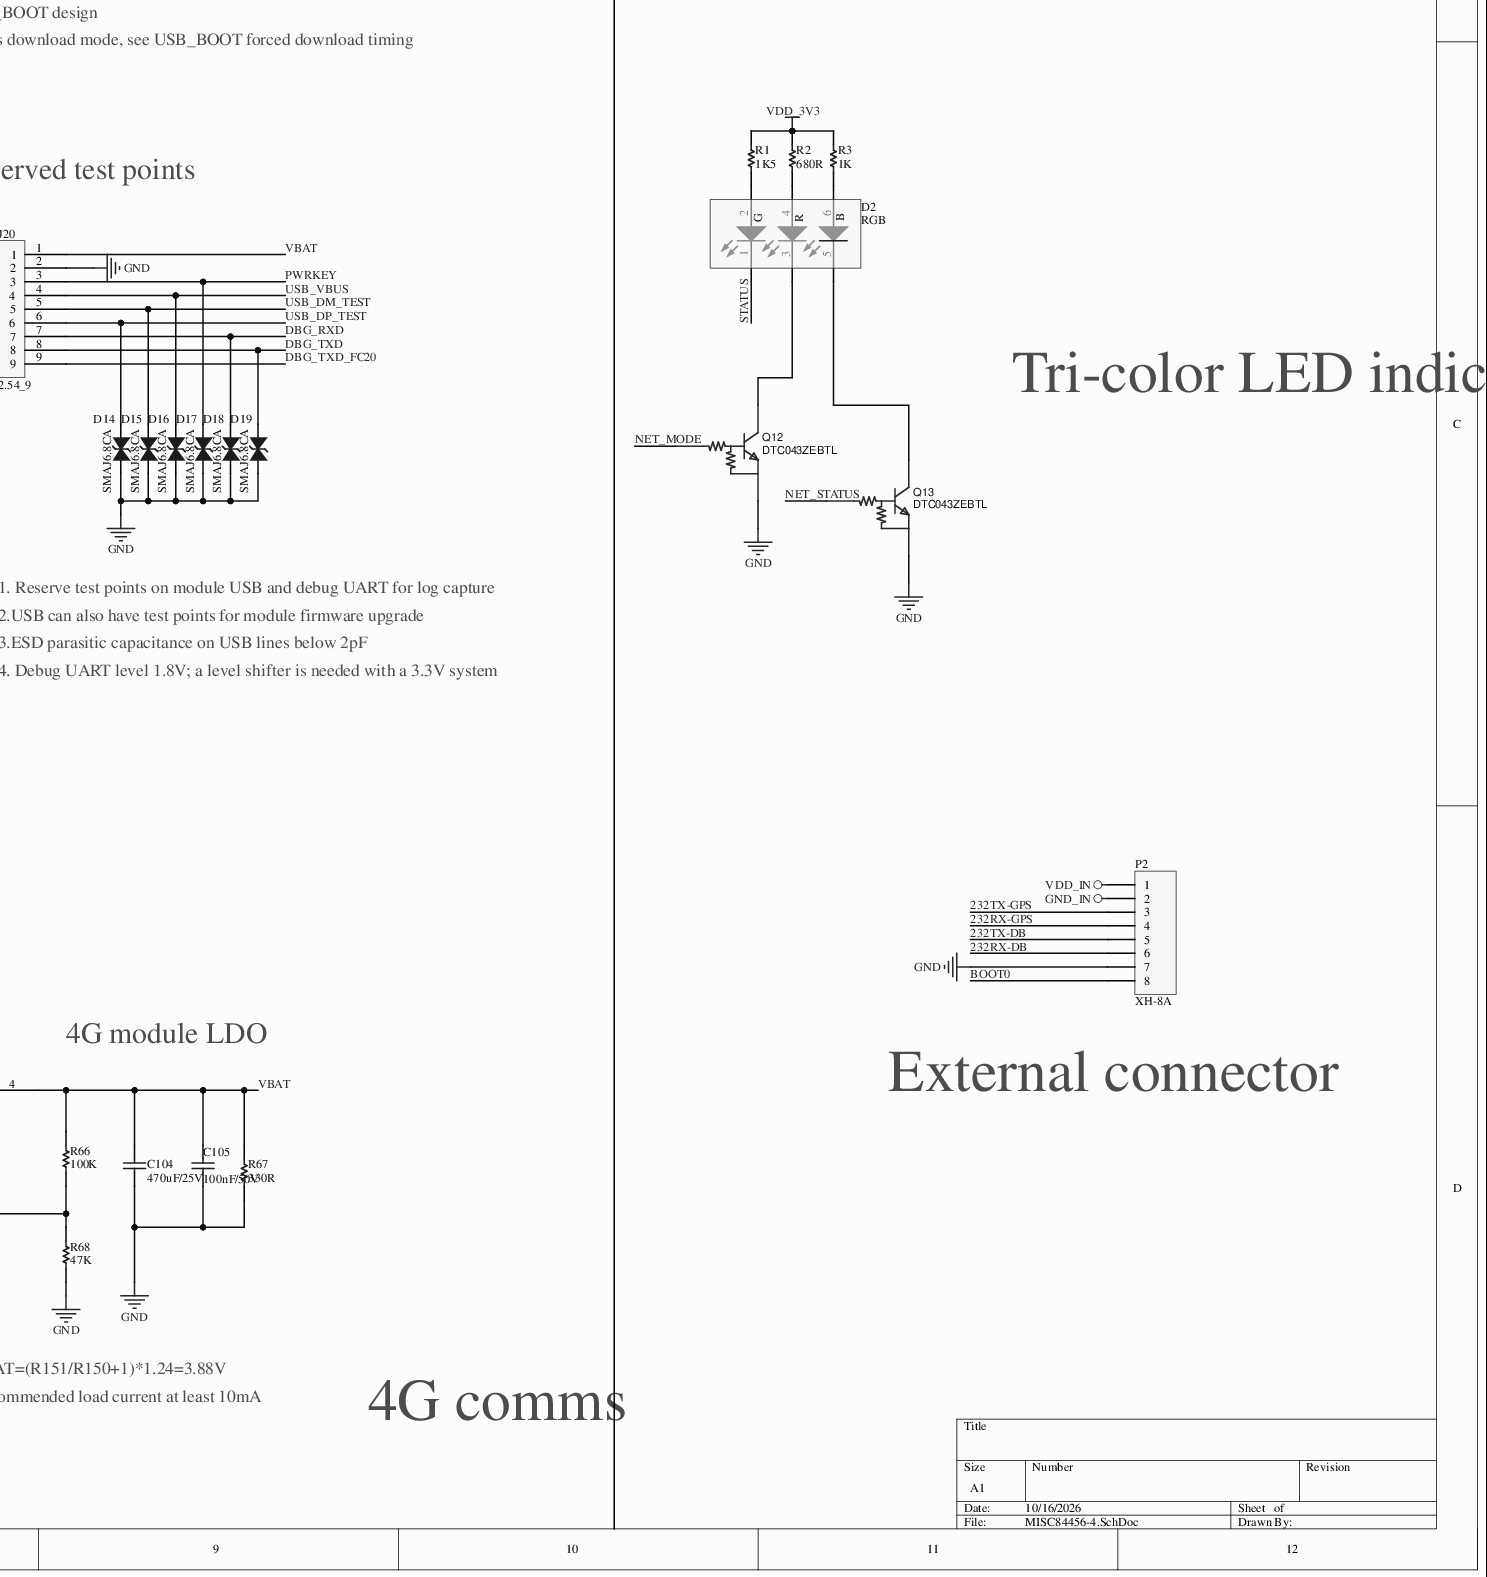
[diagram p0: MISC84456-4.SchDoc, bottom right]
# Altium project MISC84456-3.PrjPcb (part 2 of 2)

## Sheet MISC84456-4.SchDoc
size A1

### Parts
C1  100nF/50V  [C0603]
C2  100nF/50V  [C0603]
C3  100nF/50V  [C0603]  (value not drawn)
C4  470uF/25V  [RB8*11.5]
C5  10uF/25V±10%  [C1206]
C6  100nF/50V  [C0603]
C7  100pF  [C0603]
C8  100pF  [C0603]
C9  100nF/50V  [C0603]
C10  10uF/25V±10%  [C1206]
C11  100nF/50V  [C0603]  (value not drawn)
C20  100pF  [C0603]
C21  100nF/50V  [C0603]
C22  10uF/25V±10%  [C1206]
C23  100nF/50V  [C0603]
C24  100nF/50V  [C0603]
C25  100pF  [C0603]
C26  22uF/10V±20%  [C0805]
C27  100nF/50V  [C0603]
C28  22uF/10V±20%  [C0805]
C29  100uF/10V  [RB5*7]
C30  10uF/25V±10%  [C1206]
C31  100nF/50V  [C0603]
C32  10nF/50V  [C0603]
C33  100nF/50V  [C0603]
C34  33pF/50V  [C0603]
C35  33pF/50V  [C0603]
C36  33pF/50V  [C0603]
C37  33pF/50V  [C0603]
C38  100nF/50V  [C0603]
C39  100pF  [C0603]
C40  22uF/10V±20%  [C0805]
C41  100nF/50V  [C0603]
C42  22uF/10V±20%  [C0805]
C43  22uF/10V±20%  [C0805]
C44  10uF/25V±10%  [C1206]
C45  100nF/50V  [C0603]
C46  100nF/50V  [C0603]
C47  10nF/50V  [C0603]
C48  10nF/50V  [C0603]
C49  33pF/50V  [C0603]
C50  33pF/50V  [C0603]
C51  33pF/50V  [C0603]
C52  33pF/50V  [C0603]
C53  100nF/50V  [C0603]  (value not drawn)
C54  100nF/50V  [C0603]  (value not drawn)
C55  10nF/50V  [C0805]
C56  100nF/50V  [C0603]
C57  1nF/50V  [C0603]
C58  1nF/50V  [C0603]
C59  1nF/50V  [C0603]
C60  1nF/50V  [C0603]
C61  1nF/50V  [C0603]
C62  1nF/50V  [C0603]
C63  1nF/50V  [C0603]
C64  1nF/50V  [C0603]
C70  100nF/50V  [C0603]
C71  33pF/50V  [C0603]
C72  12pF/50V  [C0603]
C73  100nF/50V  [C0603]
C74  33pF/50V  [C0603]
C75  12pF/50V  [C0603]
C76  100uF/10V  [RB5*7]
C77  100uF/10V  [RB5*7]
C87  100nF/50V  [C0603]
C88  100nF/50V  [C0603]
C91  470uF/25V  [RB8*11.5]
C92  100nF/50V  [C0603]
C93  100nF/50V  [C0603]
C94  12pF/50V  [C0603]
C95  12pF/50V  [C0603]
C96  100nF/50V  [C0603]
C97  NM  [C0603]
C98  NM  [C0603]
C99  12pF/50V  [C0603]
C100  12pF/50V  [C0603]
C101  100nF/50V  [C0603]
C102  NM  [C0603]
C103  NM  [C0603]
C104  470uF/25V  [RB8*11.5]
C105  100nF/50V  [C0603]
D1  SMCJ18A  [SMC]
D2  RGB  [RGB]
D3  SMCJ18A  [SMC]
D7  GREEN  [LED0805]
D8  SMAJ6.8CA  [SMA]
D11  RGB  [RGB]
D12  RGB  [RGB]
D13  RGB  [RGB]
D14  SMAJ6.8CA  [SMA]
D15  SMAJ6.8CA  [SMA]
D16  SMAJ6.8CA  [SMA]
D17  SMAJ6.8CA  [SMA]
D18  SMAJ6.8CA  [SMA]
D19  SMAJ6.8CA  [SMA]
D24  SMAJ6.8CA  [SMA]
J1  MMCX-KE RF connector  [MMCX-KE]
J2  MMCX-KE RF connector  [MMCX-KE]
J3  UM482/K823  [UM482/K823]
J4  MMCX-KE RF connector  [MMCX-KE]
J5  POWER  [2.54mm_2x2]
J16  DLM0NSN900HY2D  [SMD_0.85x0.65mm]
J19  MMCX-KE RF connector  [MMCX-KE]
J20  2.54_9  [2.54-9P]
J21  MMCX-KE RF connector  [MMCX-KE]
J26  2.54-2  [2.54mm-2P]
K1  12V DPDT  [G6K-2P D12]
L2  120Ω ±25% @100MHz  [1812]
L3  2.2uH/2A  [SMD,4x4x2.6mm]
L4  2.2uH/2A  [SMD,4x4x2.6mm]
P1  Header 4  [HDR1X4]
P2  XH-8A  [XH-8A]
Q1  2SC4617TLQ  [SOT-416F_L1.6-W0.8-P1.00-LS1.6-TR]
Q2  8550  [SOT-23]
Q3  DTC043ZEBTL  [SOT-416_L1.6-W0.8-P1.00-LS1.6-BR]
Q4  DTC043ZEBTL  [SOT-416_L1.6-W0.8-P1.00-LS1.6-BR]
Q5  DTC043ZEBTL  [SOT-416_L1.6-W0.8-P1.00-LS1.6-BR]
Q6  DTC043ZEBTL  [SOT-416_L1.6-W0.8-P1.00-LS1.6-BR]
Q7  DTC043ZEBTL  [SOT-416_L1.6-W0.8-P1.00-LS1.6-BR]
Q8  2SC4617TLQ  [SOT-416F_L1.6-W0.8-P1.00-LS1.6-TR]
Q9  SI2333CDS-T1-E3  [SOT-23_L2.9-W1.3-P1.90-LS2.4-BR]
Q10  DTC043ZEBTL  [SOT-416_L1.6-W0.8-P1.00-LS1.6-BR]
Q11  2SC4617TLQ  [SOT-416F_L1.6-W0.8-P1.00-LS1.6-TR]
Q12  DTC043ZEBTL  [SOT-416_L1.6-W0.8-P1.00-LS1.6-BR]
Q13  DTC043ZEBTL  [SOT-416_L1.6-W0.8-P1.00-LS1.6-BR]
Q14  2SC4617TLQ  [SOT-416F_L1.6-W0.8-P1.00-LS1.6-TR]
Q15  2SC4617TLQ  [SOT-416F_L1.6-W0.8-P1.00-LS1.6-TR]
Q16  2SC4617TLQ  [SOT-416F_L1.6-W0.8-P1.00-LS1.6-TR]
Q17  2SC4617TLQ  [SOT-416F_L1.6-W0.8-P1.00-LS1.6-TR]
Q18  2SC4617TLQ  [SOT-416F_L1.6-W0.8-P1.00-LS1.6-TR]
Q19  2SC4617TLQ  [SOT-416F_L1.6-W0.8-P1.00-LS1.6-TR]
R1  1K5  [R0603]
R2  680R  [R0603]
R3  1K  [R0603]
R4  10K  [R0603]
R7  10K  [R0603]
R10  12V/2A  [R1812]
R11  75K 1%  [R0603]
R12  100K  [R0603]
R13  10K  [R0603]
R14  22R  [R0603]
R15  22R  [R0603]
R16  22R  [R0603]
R17  100K  [R0603]
R18  1K  [R0603]
R19  100K  [R0603]
R20  22.1K 1%  [R0603]
R21  22R  [R0603]
R22  NM  [R0603]
R23  22R  [R0603]
R24  22R  [R0603]
R25  10K  [R0603]
R26  0R  [R0603]
R27  0R  [R0603]
R28  0R  [R0603]
R29  10K  [R0603]
R30  4.7K  [R0603]
R31  4.7K  [R0603]
R32  0R  [R0603]
R33  NM  [R0603]
R34  NM  [R0603]
R35  10K  [R0603]
R36  10K  [R0603]
R37  10K  [R0603]
R38  10K  [R0603]
R39  4.7K  [R0603]
R40  4.7K  [R0603]
R41  10K  [R0603]
R42  NM  [R0603]
R43  4.7K  [R0603]
R44  10K  [R0603]
R45  10K  [R0603]
R46  10K  [R0603]
R47  0R  [R0603]
R48  4.7K  [R0603]
R49  10K  [R0603]
R50  0R  [R0603]
R51  4.7K  [R0603]
R52  0R  [R0603]
R53  10K  [R0603]
R54  4.7K  [R0603]
R55  10K  [R0603]
R56  4.7K  [R0603]
R57  4.7K  [R0603]
R59  4.7Ω,±1%  [R0603]
R60  4.7Ω,±1%  [R0603]
R61  4.7Ω,±1%  [R0603]
R62  0R  [R0603]
R63  4.7Ω,±1%  [R0603]
R64  0R  [R0603]
R65  47K  [R0603]
R66  100K  [R0603]
R67  330R  [R0603]
R68  47K  [R0603]
R75  1K5  [R0603]
R76  680R  [R0603]
R77  4.7K  [R0603]
R81  1K  [R0603]
R82  1K5  [R0603]
R85  1K5  [R0603]
R86  680R  [R0603]
R91  680R  [R0603]
R92  1K  [R0603]
R94  1K  [R0603]
U1  HLK-B40  [HLK-B40]
U2  24-5046-030-600-829  [HX-DU1006D]
U5  SY8113B  [TSOT-23-6]
U6  SY8113B  [TSOT-23-6]
U8  STM32F103VCT6  [LQFP-100_14x14x05P]  (parts A,B of 2)
U12  SP3232EEN  [SOP16-6.6]
U13  PESD15VL2BT  [SOT-23]
U14  PESD15VL2BT  [SOT-23]
U17  EC20  [EC20]  (parts A,B of 2)
U20  SIM-A China Telecom eSIM  [VQFN8]
U22  MIC29302WU  [TO-263-5]
U23  ESDA6V8V6-6  [SOT-563]
U24  FSA2567MPX  [MLP-16]
U25  SIM-B China Mobile eSIM  [DFN2*2-8]
U26  ESDA6V8V6-6  [SOT-563]

### Nets
ACIN: J5.3
GND: C1.1 C2.2 C3.2 C4.2 C5.1 C6.2 C7.2 C8.1 C9.1 C10.1 C11.2 C20.1 C21.1 C22.1 C24.2 C26.2 C27.2 C28.2 C29.2 C30.1 C31.1 C32.2 C34.2 C35.2 C36.2 C37.2 C38.1 C40.2 C41.2 C42.2 C43.2 C44.1 C45.2 C46.1 C47.2 C48.2 C49.2 C50.2 C51.2 C52.2 C53.2 C54.2 C55.1 C56.2 C70.2 C71.2 C72.2 C73.2 C74.2 C75.2 C76.2 C77.2 C88.2 C91.2 C92.2 C94.1 C95.1 C96.2 C97.1 C98.1 C99.2 C100.2 C101.2 C102.1 C103.1 C104.2 C105.2 D3.1(A) D7.2(K) D8.1(A) D14.1(A) D15.1(A) D16.1(A) D17.1(A) D18.1(A) D19.1(A) D24.1(A) J1.2 J1.3 J1.4 J1.5 J2.2 J2.3 J2.4 J2.5 J3.1(GND10) J3.3(GND11) J3.4(GND12) J3.6(GND13) J3.9(GND14) J3.14(GND15) J3.18(GND16) J3.25(GND17) J3.33(GND1) J3.34(GND2) J3.43(GND3) J3.47(GND4) J3.52(GND5) J3.55(GND6) J3.57(GND7) J3.58(GND8) J3.60(GND9) J4.2 J4.3 J4.4 J4.5 J5.2 J19.2 J19.3 J19.4 J19.5 J20.2 J21.2 J21.3 J21.4 J21.5 L2.2 P1.3 P2.7 Q3.2(E) Q4.2(E) Q5.2(E) Q6.2(E) Q7.2(E) Q10.2(E) Q12.2(E) Q13.2(E) Q19.1(E) R4.1 R7.2 R13.1 R20.1 R36.1 R42.1 R67.1 R68.1 U1.1(GND) U1.10(GND) U1.28(GND) U2.1(GND) U2.5(GND) U2.7(GND) U2.9(GND) U2.19(GND) U2.20(GND) U2.21(GND) U2.22(GND) U2.30(GND) U5.2(GND) U6.2(GND) U8.10(VSS_5) U8.19(VSSA) U8.20(VREF-) U8.27(VSS_4) U8.49(VSS_1) U8.74(VSS_2) U8.99(VSS_3) U12.15(GND) U13.3 U14.3 U17.8(GND) U17.9(GND) U17.19(GND) U17.22(GND) U17.36(GND) U17.46(GND) U17.48(GND) U17.50(GND) U17.51(GND) U17.52(GND) U17.53(GND) U17.54(GND) U17.56(GND) U17.72(GND) U17.85(GND) U17.86(GND) U17.87(GND) U17.88(GND) U17.89(GND) U17.90(GND) U17.91(GND) U17.92(GND) U17.93(GND) U17.94(GND) U17.95(GND) U17.96(GND) U17.97(GND) U17.98(GND) U17.99(GND) U17.100(GND) U17.101(GND) U17.102(GND) U17.103(GND) U17.104(GND) U17.105(GND) U17.106(GND) U17.107(GND) U17.108(GND) U17.109(GND) U17.110(GND) U17.111(GND) U17.112(GND) U20.1(GND) U22.3(GND) U23.2 U24.6(GND) U25.1(GND) U26.2
GND_IN: L2.1 P2.2
VDD_3V3: C2.1 C3.1 C11.1 C20.2 C21.2 C22.2 C38.2 C39.1 C40.1 C41.1 C42.1 C43.1 C53.1 C54.1 C55.2 C56.1 C88.1 J3.31(VCC1) J3.32(VCC2) J5.4 L4.2 Q2.2(E) R1.1 R2.1 R3.1 R17.2 R18.1 R25.2 R35.2 R38.2 R46.2 R49.2 R53.2 R55.2 R75.1 R76.1 R81.1 R82.1 R85.1 R86.1 R91.1 R92.1 R94.1 U1.9(VBAT) U2.18(3V3) U2.23(3V3) U2.24(3V3) U2.25(3V3) U2.26(3V3) U2.27(3V3) U2.28(3V3) U8.11(VDD_5) U8.21(VREF+) U8.22(VDDA) U8.28(VDD_4) U8.50(VDD_1) U8.75(VDD_2) U8.100(VDD_3) U12.16(VCC) U24.14(VCC)
VDD_5V: C5.2 C6.1 C7.1 C8.2 C9.2 C10.2 C25.1 C26.1 C27.1 C28.1 C29.1 C91.1 C101.1 J3.5(ANT1_PWR) J3.56(ANT2_PWR) L3.2 Q9.2(S) R11.2 R29.1 R65.2 U22.2(IN)
VDD_12V: C4.1 C30.2 C31.2 C44.2 C46.2 D1.2(K) D3.2(K) K1.1(VCC) R10.1 R12.2 R19.2 U5.5(VIN) U6.5(VIN)
VDD_EXT: C57.1 C58.2 C59.1 C60.1 C61.2 C62.2 C63.2 C64.2 R30.1 R31.1 R39.2 R40.2 R41.1 R43.2 R44.1 R45.1 R48.1 R51.1 R54.1 R56.1 R77.1 U17.7(VDD_EXT)
VDD_IN: J5.1 P2.1 R10.2
232RX-DB: P2.6 R63.1 U14.1
232RX-GPS: P2.4 R60.1 U13.1
232TX-DB: P2.5 R61.1 U14.2
232TX-GPS: P2.3 R59.1 U13.2
433_CH_SW: R57.2 U8.16(PC1/ADC_IN11)
433_M0: U2.11(CONFIG) U8.17(PC2/ADC_IN12)
433_RTK_RX: J3.37(TXD2) K1.2
433_RTK_TX: J3.38(RXD2) K1.7
433_RX: K1.3 U2.3(RXD)
433_SIGNAL: U2.12(RSSI) U8.23(PA0-WKUP/USART2_CTS/ADC_IN0/TIM2_CH1_ETR)
433_SW: U2.13(T/~{RX}_SW) U8.15(PC0/ADC_IN10)
433_TX: K1.6 U2.14(TXD)
ANT_DIV: C103.2 R64.1 U17.35(ANT_DIV)
ANT_GNSS: U17.47(ANT_GNSS)
ANT_MAIN: C98.2 R62.1 U17.49(ANT_MAIN)
AP_READY_MODULE: Q8.3(C) R30.2 U17.2(AP_READY)
BLE_RST: U1.7(RESET) U8.40(PE9)
BLE_SLP: U1.17(PC6) U8.38(PE7)
BLE_SW: U1.18(PC5) U8.39(PE8)
BOOT0: P2.8 R37.2 R38.1
CPU-URX0: U8.69(PA10/USART1_RX/TIM1_CH3) U12.9(R2OUT)
CPU-UTX0: U8.68(PA9/USART1_TX/TIM1_CH2) U12.10(T2IN)
DBG_RXD: D18.2(K) J20.7 U17.11(DBG_RXD)
DBG_TXD: D19.2(K) J20.8 U17.12(DBG_TXD)
DBG_TXD_FC20: J20.9
GPS_RXD1: J3.36(RXD1) U12.12(R1OUT)
GPS_TXD1: J3.35(TXD1) U12.11(T1IN)
JTCK: P1.1 R7.1 U8.76(PA14/JTCK-SWCLK)
JTMS: P1.2 R25.1 U8.72(PA13/JTMS-SWDAT)
LED1_B: D11.5(K) U8.41(PE10)
LED1_G: D11.1(K) U8.43(PE12)
LED1_R: D11.3(K) U8.42(PE11)
LED2_B: D12.5(K) U8.44(PE13)
LED2_G: D12.1(K) U8.46(PE15)
LED2_R: D12.3(K) U8.45(PE14)
LED3_B: D13.5(K) U1.25(PA4)
LED3_G: D13.1(K) U1.16(PC7)
LED3_R: D13.3(K) U1.26(PA5)
NET_MODE: Q12.1(B) U17.5(NET_MODE)
NET_STATUS: Q13.1(B) U17.6(NET_STATUS)
NRST: C1.2 P1.4 R35.1 U8.14(NRST)
ON/OFF_MCU: Q3.1(B) U8.59(PD12)
PB2_BOOT1: R4.2 U8.37(PB2_/_BOOT1)
PWRKEY: C32.1 D17.2(K) J20.3 Q3.3(C) U17.21(PWRKEY)
RESET_MCU: Q4.1(B) U8.56(PD9)
RESET_N: Q4.3(C) U17.20(RESET_N)
SIM_SEL: R22.1 U8.62(PD15) U24.2(SEL)
SIMA_CLK: R15.1 U24.9(1CLK)
SIMA_DATA: R16.1 U24.13(1DAT)
SIMA_RST: R14.1 U24.5(1RST)
SIMA_VDD: C24.1 C34.1 U20.8(VCC) U23.1 U24.1(1VSIM)
SIMB_CLK: R23.1 U24.7(2CLK)
SIMB_DATA: R24.1 U24.11(2DAT)
SIMB_RST: R21.1 U24.3(2RST)
SIMB_VDD: C45.1 C49.1 U24.15(2VSIM) U25.8(VCC) U26.1
SLEEP_STATUS: Q8.1(E) U8.55(PD8)
STATUS: D2.1(K) U17.61(STATUS)
UART2_RXD: U1.23(UART0-TX) U8.26(PA3/USART2_RX/ADC_IN3/TIM2_CH4)
UART2_TXD: U1.24(UART0-RX) U8.25(PA2/USART2_TX/ADC_IN2/TIM2_CH3)
UART3_CTS: Q14.3(C) R46.1 U8.52(PB13/SPI2_SCK/USART3_CTS/TIM1_CH1N)
UART3_DCD: Q17.3(C) R53.1 U8.95(PB8/TIM4_CH3)
UART3_DTR: Q15.1(E) U8.51(PB12/SPI2_NSS/I2C2_SMBAl/USART3_CK/TIM1_BKIN)
UART3_RI: Q18.3(C) R55.1 U8.96(PB9/TIM4_CH4)
UART3_RTS: Q1.1(E) U8.53(PB14/SPI2_MISO/USART3_RTS/TIM1_CH2N)
UART3_RXD: Q16.3(C) R49.1 U8.48(PB11/I2C2_SDA_/USART3_RX)
UART3_TXD: Q11.1(E) U8.47(PB10/I2C2_SCL/USART3_TX)
UART4_RXD: J3.39(TXD3) U8.79(PC11)
UART4_TXD: J3.40(RXD3) U8.78(PC10)
UART5_RXD: K1.5 U8.83(PD2/TIM3_ETR)
UART5_TXD: K1.4 U8.80(PC12)
USB-DM2: J16.4 U8.70(PA11/USART1_CTS/CANRX/USBDM_(2)/TIM1_CH4)
USB-DP2: J16.1 U8.71(PA12/USART1_RTS/CANTX/USBDP_(2)/TIM1_ETR)
USB_BOOT: D24.2(K) J26.2 U17.115(USB_BOOT)
USB_DM_TEST: D15.2(K) J20.5 R34.1
USB_DP_TEST: D14.2(K) J20.6 R33.1
USB_VBUS: D16.2(K) J20.4 Q9.3(D) U17.71(USB_VBUS)
USIM_CLK: U17.16(USIM_CLK) U24.8(CLK)
USIM_DATA: U17.15(USIM_DATA) U24.12(DAT)
USIM_GND: U17.10(USIM_GND)
USIM_PRESENCE: R42.2 U17.13(USIM_PRESENCE)
USIM_RST: U17.17(USIM_RST) U24.4(RST)
USIM_VDD: U17.14(USIM_VDD) U24.16(VSIM)
VBAT: C70.1 C71.1 C72.1 C73.1 C74.1 C75.1 C76.1 C77.1 C104.1 C105.1 D8.2(K) J20.1 R66.2 R67.2 U17.57(VBAT_RF) U17.58(VBAT_RF) U17.59(VBAT_BB) U17.60(VBAT_BB) U22.4(OUT)
VBAT_EN: Q10.1(B) U8.60(PD13)
VBUS_CTRL: Q7.1(B) U8.61(PD14)
W_DISABLE_MCU: Q6.1(B) U8.57(PD10)
W_DISABLE_MODULE: C48.1 Q6.3(C) U17.4(W_DISABLE#)
WAKEUP_IN_MCU: Q5.1(B) U8.58(PD11)
WAKEUP_IN_MODULE: C47.1 Q5.3(C) U17.1(WAKEUP_IN)
XTAL1: U8.12(OSC_IN)
NetC23_1: C23.1 L3.1 U5.6(LX)
NetC23_2: C23.2 U5.1(BS)
NetC25_2: C25.2 R11.1 R13.2 U5.3(FB/OUT)
NetC33_1: C33.1 L4.1 U6.6(LX)
NetC33_2: C33.2 U6.1(BS)
NetC35_1: C35.1 R14.2 U20.7(RST) U23.3
NetC36_1: C36.1 R15.2 U20.6(CLK) U23.6
NetC37_1: C37.1 R16.2 U20.3(I/O) U23.5
NetC39_2: C39.2 R17.1 R20.2 U6.3(FB/OUT)
NetC50_1: C50.1 R21.2 U25.7(RST) U26.3
NetC51_1: C51.1 R23.2 U25.6(CLK) U26.5
NetC52_1: C52.1 R24.2 U25.3(I/O) U26.4
NetC57_2: C57.2 Q1.2(B) R39.1
NetC58_1: C58.1 Q8.2(B) R31.2
NetC59_2: C59.2 Q11.2(B) R40.1
NetC60_2: C60.2 Q15.2(B) R43.1
NetC61_1: C61.1 Q14.2(B) R48.2
NetC62_1: C62.1 Q16.2(B) R51.2
NetC63_1: C63.1 Q17.2(B) R54.2
NetC64_1: C64.1 Q18.2(B) R56.2
NetC87_1: C87.1 U12.3(C1-)
NetC87_2: C87.2 U12.1(C1+)
NetC92_1: C92.1 U12.2(V+)
NetC93_1: C93.1 U12.5(C2-)
NetC93_2: C93.2 U12.4(C2+)
NetC94_2: C94.2 R59.2 U12.14(T1OUT)
NetC95_2: C95.2 R60.2 U12.13(R1IN)
NetC96_1: C96.1 U12.6(V-)
NetC97_2: C97.2 J19.1 R62.2
NetC99_1: C99.1 R63.2 U12.8(R2IN)
NetC100_1: C100.1 R61.2 U12.7(T2OUT)
NetC102_2: C102.2 J21.1 R64.2
NetD1_1: D1.1(A) K1.8 Q19.3(C)
NetD2_2: D2.2(A) R1.2
NetD2_3: D2.3(K) Q12.3(C)
NetD2_4: D2.4(A) R2.2
NetD2_5: D2.5(K) Q13.3(C)
NetD2_6: D2.6(A) R3.2
NetD7_1: D7.1(A) R18.2
NetD11_2: D11.2(A) R75.2
NetD11_4: D11.4(A) R76.2
NetD11_6: D11.6(A) R81.2
NetD12_2: D12.2(A) R82.2
NetD12_4: D12.4(A) R86.2
NetD12_6: D12.6(A) R92.2
NetD13_2: D13.2(A) R85.2
NetD13_4: D13.4(A) R91.2
NetD13_6: D13.6(A) R94.2
NetJ1_1: J1.1 J3.2(ANT1_IN)
NetJ2_1: J2.1 U1.29(ANT)
NetJ3_59: J3.59(ANT2_IN) J4.1
NetJ16_2: J16.2 R33.2 U17.69(USB_DP)
NetJ16_3: J16.3 R34.2 U17.70(USB_DM)
NetJ26_1: J26.1 R77.2
NetQ1_3: Q1.3(C) R26.1 R41.2
NetQ2_1: Q2.1(B) R37.1
NetQ2_3: Q2.3(C) R36.2 U8.94(BOOT0)
NetQ7_3: Q7.3(C) Q9.1(G) R29.2
NetQ10_3: Q10.3(C) R65.1 U22.1(EN)
NetQ11_3: Q11.3(C) R32.1 R44.2
NetQ14_1: Q14.1(E) R47.1
NetQ15_3: Q15.3(C) R27.1 R45.2
NetQ16_1: Q16.1(E) R28.1
NetQ17_1: Q17.1(E) R50.1
NetQ18_1: Q18.1(E) R52.1
NetQ19_2: Q19.2(B) R57.1
NetR12_1: R12.1 U5.4(EN)
NetR19_1: R19.1 U6.4(EN)
NetR22_2: R22.2 U24.10(NC)
NetR26_2: R26.2 U17.65(RTS)
NetR27_2: R27.2 U17.66(DTR)
NetR28_2: R28.2 U17.67(TXD)
NetR32_2: R32.2 U17.68(RXD)
NetR47_2: R47.2 U17.64(CTS)
NetR50_2: R50.2 U17.63(DCD)
NetR52_2: R52.2 U17.62(RI)
NetR66_1: R66.1 R68.2 U22.5(ADJ)

Not connected (* = marked no-connect by the designer): J3 7(ANT1_NLOD) 8(ANT1_FFLG) 10(RSV5) 11(RSV6) 12(RSV7) 13(RSV8) 15(SPEED) 16(FWR) 17(VBAT) 19(GPIO1) 20(GPIO2) 21(RSV9) 22(FRESET) 23(ERR_STAT) 24(RTK_STAT) 26(SPI_MISO) 27(SPI_MOSI) 28(SPI_CLK) 29(SS0) 30(SS1) 41(I2C_SDA) 42(I2C_SCL) 44(PPS) 45(EVENT) 46(RST) 48(RSV1) 49(RSV2) 50(RSV3) 51(RSV4) 53(ANT2_FFLG) 54(ANT2_NLOD); U1 2(MIC-BIAS) 3(MIC-IN) 4(VMID) 5(AOUT-P) 6(AOUT-N) 8(VCHG) 11(VDDIO) 12(PD7) 13(PD6) 14(PD5) 15(PD4) 19(PA3) 20(PA2) 21(PA1) 22(PA0) 27(LED); U2 6(RX_CLK) 8(TX_CLK); U8 1(PE2) 2(PE3) 3(PE4) 4(PE5) 5(PE6) 6(VBAT) 7(PC13-ANTI_TAMP) 8(PC14-OSC32_IN) 9(PC15-OSC32_OUT) 13(OSC_OUT) 18(PC3/ADC_IN13) 24(PA1/USART2_RTS/ADC_IN1/TIM2_CH2) 29(PA4/SPI1_NSS/USART2_CK/ADC_IN4) 30(PA5/SPI1_SCK/ADC_IN5) 31(PA6/SPI1_MISO/ADC_IN6/TIM3_CH1) 32(PA7/SPI1_MOSI/ADC_IN7/TIM3_CH2) 33(PC4/ADC_IN14) 34(PC5/ADC_IN15) 35(PB0/ADC_IN8/TIM3_CH3) 36(PB1/ADC_IN9/TIM3_CH4) 54(PB15/SPI2_MOSI/TIM1_CH3N) 63(PC6) 64(PC7) 65(PC8) 66(PC9) 67(PA8/USART1_CK/TIM1_CH1/MCO) 73(Not_connected) 77(PA15/JTDI) 81(PD0) 82(PD1) 84(PD3) 85(PD4) 86(PD5) 87(PD6) 88(PD7) 89(PB3/JTDO) 90(PB4/JTRST) 91(PB5/I2C1_SMBAl) 92(PB6/I2C1_SCL/TIM4_CH1) 93(PB7/I2C1_SDA/TIM4_CH2) 97(PE0/TIM4_ETR) 98(PE1); U17 3(RVD) 18(RVD) 23(SD_INS_DET) 24(PCM_IN) 25(PCM_OUT) 26(PCM_SYNC) 27(PCM_CLK) 28(SDC2_DATA3) 29(SDC2_DATA2) 30(SDC2_DATA1) 31(SDC2_DATA0) 32(SDC2_CLK) 33(SDC2_CMD) 34(VDD_SDIO) 37(BT_RTS) 38(BT_TXD) 39(BT_RXD) 40(BT_CTS) 41(I2C_SCL) 42(I2C_SDA) 43(RVD) 44(ADC1) 45(ADC0) 55(RVD) 113(RVD) 114(RVD) 116(RVD) 117(RESERVED) 118(WLAN_SLP_CLK) 119(EPHY_RST_N) 120(EPHY_INT_N) 121(SGMII_MDATA) 122(SGMII_MCLK) 123(SGMII_TX_M) 124(SGMII_TX_P) 125(SGMII_RX_P) 126(SGMII_RX_M) 127(PM_ENABLE) 128(USIM2_VDD) 129(SDC1_DATA3) 130(SDC1_DATA2) 131(SDC1_DATA1) 132(SDC1_DATA0) 133(SDC1_CLK) 134(SDC1_CMD) 135(WAKE_ON_WIRELESS) 136(WLAN_EN) 137(COEX_UART_RX) 138(COEX_UART_TX) 139(BT_EN) 140(RESERVED) 141(RVD) 142(RVD) 143(RVD) 144(RVD); U20 2(NC) 4(NC) 5(NC); U23 4; U25 2(NC) 4(NC) 5(NC); U26 6

### Notes on the sheet
- 12V
- 5V
- 433_Radio
- (near U2) M0=0 transparent mode
- M0=1 config mode
- GPS
- 3V3
- (near R37) Active low
- MCU
- RS232-DEBUG
- Bluetooth
- USB_BOOT
- 1. Strongly recommend reserving the USB_BOOT design
- 2.USB_BOOT floats by default; high forces download mode, see USB_BOOT forced download timing
- Reserved test points
- Tri-color LED indicator
- 1. Reserve test points on module USB and debug UART for log capture
- 2.USB can also have test points for module firmware upgrade
- Main antenna
- 3.ESD parasitic capacitance on USB lines below 2pF
- 4. Debug UART level 1.8V; a level shifter is needed with a 3.3V system
- 1. Leave all unused and RESERVED pins floating; connect all GND pins to the ground net
- 2. Pins 73-84 are for internal use: no schematic or footprint design needed; no copper pour or routing in this area
- 3. Put common-mode inductor L0101 in series on the MCU-module USB link to filter EMI; place it close to the module
- (near Q3) Module power on/off
- (near Q4) Module reset
- Also reserve USB upgrade test points, keep stubs short, place the 2 resistors near the module USB port for signal integrity
- 4.ADC pins must not connect directly to module power; input voltage must not exceed VBAT_BB
- 5.Place C0101 and C0102 near the module SGMII receive port (not connected)
- Diversity antenna
- 6. WAKEUP_IN, NET_MODE, BT_CTS, COEX_UART_TX, COEX_UART_RX and WLAN_EN must not be pulled up before the module boots
- 7.EC25/EC21/EC20 R2.1/EG25-G used with FC20: connect EC25/EC21/EC20 R2.1/EG25-G BT_UART and PCM to FC20 BT_UART and BT_PCM
- 4G module LDO
- (near Q6) Module airplane mode
- Near VBAT_BB
- Near VBAT_RF
- External connector
- Module wakeup
- 1. Reserve PI networks for main, diversity and FC20 antennas for later tuning
- 2. Diversity receive is on by default; if unused, disable it by AT command; for AT command details,
- 3. An active GNSS antenna needs the VDD supply circuit; with a passive antenna it may be left unpopulated.
- See Quectel_EC25/EC21/EC20 R2.1/EG25-G/EG21-G/EG20-CN Hardware Design manual
- Choose GNSS supply VDD per the active antenna requirements
- 4. RF antenna single-ended impedance is 50Ω
- 5.EC20-CN has no Bluetooth, WIFI or GNSS: no GNSS or FC20 antenna circuit
- VBAT supply must deliver a rated 2.0A
- VBAT=(R151/R150+1)*1.24=3.88V
- 6.EG21-G has no Bluetooth or WIFI: no FC20 antenna circuit
- Route VBAT in a star to pins VBAT_BB and VBAT_RF
- VBAT operating range 3.3V-4.3V
- Recommended load current at least 10mA
- 4G comms

### Library data of the parts
C1-C3 C11 C53-C56 = Cap: SMD capacitor; Published: 8-Jun-2000; Revision: July-2002: Re-released for DXP Platform.; Publisher: Altium Limited
  C1-C3 C11 C53 C54 C56: Value: 100nF/50V
  C55: Value: 10nF/50V
C4 C91 C104 = Cap: 470μF,25V,Ф8×11.5mm,RoHS; Published: 8-Jun-2000; LatestRevisionDate: 17-Jul-2002; LatestRevisionNote: Re-released for DXP Platform.; PackageReference: RAD-0.3; Value: 470uF/25V; Publisher: Altium Limited
C5 C10 C22 C30 C44 = Cap: SMD ceramic capacitor,X7R; Published: 8-Jun-2000; LatestRevisionDate: 17-Jul-2002; LatestRevisionNote: Re-released for DXP Platform.; PackageReference: RAD-0.3; Value: 10uF/25V±10%; Publisher: Altium Limited
C6-C9 C20 C21 C23-C25 C27 C31-C39 C41 C45-C52 C57-C64 C70-C75 C97 C98 C101-C103 C105 = Cap: SMD ceramic capacitor; Published: 8-Jun-2000; LatestRevisionDate: 17-Jul-2002; LatestRevisionNote: Re-released for DXP Platform.; PackageReference: RAD-0.3; Publisher: Altium Limited
  C6 C9 C21 C23 C24 C27 C31 C33 C38 C41 C45 C46 C70 C73 C101 C105: Value: 100nF/50V
  C7 C8 C20 C25 C39: Value: 100pF
  C32 C47 C48: Value: 10nF/50V
  C34-C37 C49-C52 C71 C74: Value: 33pF/50V
  C57-C64: Value: 1nF/50V
  C72 C75: Value: 12pF/50V
  C97 C98 C102 C103: Value: NM
C26 C28 C40 C42 C43 = Cap: SMD ceramic capacitor,X5R; Published: 8-Jun-2000; LatestRevisionDate: 17-Jul-2002; LatestRevisionNote: Re-released for DXP Platform.; PackageReference: RAD-0.3; Value: 22uF/10V±20%; Publisher: Altium Limited
C29 C76 C77 = Cap2: 100μF,10V,Ф5×7mm,RoHS; Published: 23-Sep-2002; PackageReference: CAPR5-4X5; Value: 100uF/10V; Publisher: Altium Limited
C87 C88 C92-C96 C99 C100 = Cap: SMD capacitor,X7R; Published: 8-Jun-2000; Revision: July-2002: Re-released for DXP Platform.; Publisher: Altium Limited
  C87 C88 C92 C93 C96: Value: 100nF/50V
  C94 C95 C99 C100: Value: 12pF/50V
D1 D3 = Diode: Default Diode; Published: 8-Jun-2000; LatestRevisionDate: 17-Jul-2002; LatestRevisionNote: Re-released for DXP Platform.; PackageVersion: Sep-1996; PackageReference: SMC; Code_JEDEC: DO-214-AB; Publisher: Altium Limited
D2 D11-D13 = LED1_3: Full-color RGB LED,19-337C/RSBHGHC-M03/2T; Published: 8-Jun-2000; LatestRevisionDate: 08-Jul-2005; LatestRevisionNote: Mech Layer 1 removed.; PackageReference: LED-1; Publisher: Altium Limited
D7 = LED1: Typical RED GaAs LED; Published: 8-Jun-2000; LatestRevisionDate: 08-Jul-2005; LatestRevisionNote: Mech Layer 1 removed.; PackageReference: LED-1; Publisher: Altium Limited
D8 D14-D19 D24 = Diode_1: SMD TVS diode; Published: 8-Jun-2000; LatestRevisionDate: 17-Jul-2002; LatestRevisionNote: Re-released for DXP Platform.; PackageVersion: Sep-1996; PackageReference: SMC; Code_JEDEC: DO-214-AB; Publisher: Altium Limited
J1 J2 J4 J19 J21 = CIRCLE
J3 = UM482
J5 = 2.54
K1 = Relay-DPDT: G6K-2P D12,OMRON; Published: 24-Mar-1999; LatestRevisionDate: 17-Jul-2002; LatestRevisionNote: Re-released for DXP Platform.; PackageReference: DIP-P8; PackageDescription: Relay; 8 Leads; Publisher: Altium Limited
L2 = Inductor: Ferrite bead; Code_IEC: 1005; Published: 8-Jun-2000; LatestRevisionDate: 29-May-2009; LatestRevisionNote: IPC-7351 Footprint Added.; PackageReference: 0402-A; PackageDescription: Chip Inductor; Code_JEITA: 0402; Publisher: Altium Limited
L3 L4 = Inductor: SMD power inductor,cjiang(Changjiang Micro),FNR4026S2R2MT; Code_IEC: 1005; Published: 8-Jun-2000; LatestRevisionDate: 29-May-2009; LatestRevisionNote: IPC-7351 Footprint Added.; PackageReference: 0402-A; PackageDescription: Chip Inductor; Code_JEITA: 0402; Value: 2.2uH/2A; Publisher: Altium Limited
P1 = Header 4: Header, 4-Pin; LatestRevisionDate: 17-Jul-2002; LatestRevisionNote: Re-released for DXP Platform.; Publisher: Altium Limited
P2 = Header 8: Header, 8-Pin; LatestRevisionDate: 17-Jul-2002; LatestRevisionNote: Re-released for DXP Platform.; Publisher: Altium Limited
Q1 Q8 Q11 Q14-Q19 = 2SC4617TLQ: BOM_Manufacturer: ROHM Semicon; Contributor: LCSC; BOM_Supplier: LCSC; BOM_Supplier Part: C308648; BOM_Manufacturer Part: 2SC4617TLQ; spicePre: Q; spiceSymbolName: 2SC4617TLQ
Q2 = PNP: PNP Bipolar Transistor; Published: 8-Jun-2000; LatestRevisionDate: 29-May-2009; LatestRevisionNote: IPC-7351 Footprint Added.; PackageVersion: Aug-1999; PackageReference: SOT-23B; PackageDescription: 3-Pin SOT-23 Package 0.95 mm Pitch, 2.4 mm Lead Span; Publisher: Altium Limited
Q3-Q7 Q10 Q12 Q13 = DTC043ZEBTL: BOM_Manufacturer: ROHM; BOM_Paste Type: expand; BOM_Supplier: LCSC; BOM_Manufacturer Part: DTC043ZEBTL; BOM_Supplier Part: C96459; spicePre: Q; spiceSymbolName: DTC043ZEBTL
Q9 = SI2333CDS-T1-E3: BOM_Manufacturer: VISHAY; Contributor: LCSC; BOM_Paste Type: expand; BOM_Supplier: LCSC; BOM_Manufacturer Part: SI2333CDS-T1-E3; BOM_Supplier Part: C144846; spicePre: Q; spiceSymbolName: SI2333CDS-T1-E3
R1-R3 R18 R41 R44-R46 R49 R53 R55 R75 R76 R81 R82 R85 R86 R91 R92 R94 = Res1: SMD resistor; Published: 8-Jun-2000; LatestRevisionDate: 17-Jul-2002; LatestRevisionNote: Re-released for DXP Platform.; PackageReference: AXIAL-0.3; Publisher: Altium Limited
  R1 R75 R82 R85: Value: 1K5
  R2 R76 R86 R91: Value: 680R
  R3 R18 R81 R92 R94: Value: 1K
  R41 R44-R46 R49 R53 R55: Value: 10K
R4 R35-R38 = Res: SMD resistor; Published: 8-Jun-2000; LatestRevisionDate: 04-Mar-2005; LatestRevisionNote: PCB Footprint replaced.; PackageReference: J1-0603; Value: 10K; Publisher: Altium Limited
R7 R11-R17 R19-R34 R39 R40 R42 R43 R47 R48 R50-R52 R54 R56 R57 R62 R64-R68 R77 = Res1: Resistor; Published: 8-Jun-2000; LatestRevisionDate: 17-Jul-2002; LatestRevisionNote: Re-released for DXP Platform.; PackageReference: AXIAL-0.3; Publisher: Altium Limited
  R7 R13 R25 R29: Value: 10K
  R11: Value: 75K 1%
  R12 R17 R19 R66: Value: 100K
  R14-R16 R21 R23 R24: Value: 22R
  R20: Value: 22.1K 1%
  R22 R33 R34 R42: Value: NM
  R26-R28 R32 R47 R50 R52 R62 R64: Value: 0R
  R30 R31 R39 R40 R43 R48 R51 R54 R56 R57 R77: Value: 4.7K
  R65 R68: Value: 47K
  R67: Value: 330R
R10 = RES: Resettable fuse
R59-R61 R63 = RES: SMD resistor; Value: 4.7Ω,±1%
U1 = HLK-B40: BLE5.1 Bluetooth module,Shenzhen Hi-Link
U2 = HX-DU1006D: Kyocera Japan, 5046 series, mates HX-DU1006D
U8 = STM32F103VBH6: Integrated IC
U12 = SP202ECT
U13 U14 = PESD12VL2BT
U17 = EC25/EC21
U20 U25 = SIM-A
U24 = FSA2567